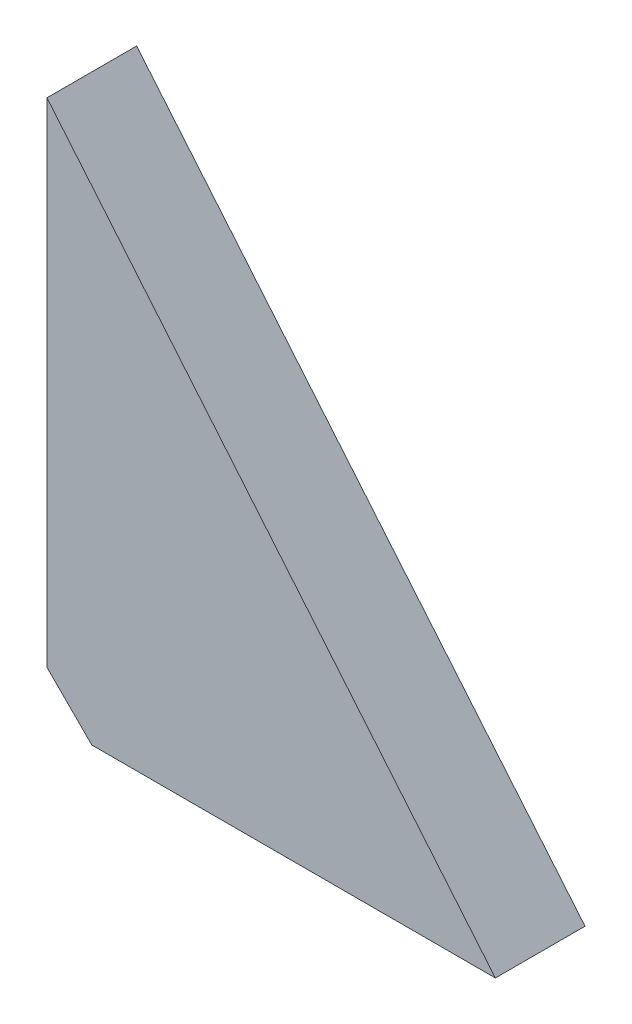
from build123d import *

# Parameters (mm, degrees)
BOSS_EXTRUDE1_DEPTH = 5
CHAMFER1_SIZE       = 5


with BuildPart() as part:
    # Sketch1 → Boss-Extrude1 (new, symmetric)
    with BuildSketch(Plane.XY):
        Polygon((0, 0), (0, 60), (50, 0), align=None)
    extrude(amount=BOSS_EXTRUDE1_DEPTH, both=True)

    # Chamfer1
    chamfer1_edges = [part.edges().sort_by_distance(p)[0] for p in [
        (0, 0, 0),
    ]]
    chamfer(chamfer1_edges, length=CHAMFER1_SIZE)


solid = part.part
